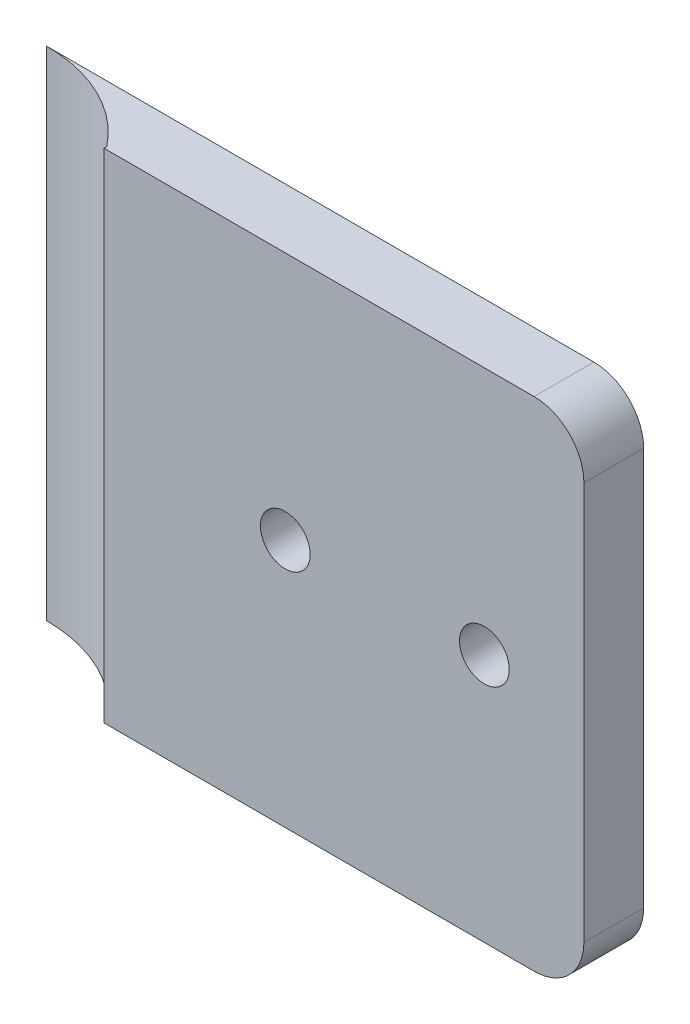
from build123d import *

# Parameters (mm, degrees)
BOSS_EXTRUDE1_DEPTH   = 6
BOSS_EXTRUDE2_DEPTH   = 50
M6_TAPPED_HOLE1_D     = 5
M6_TAPPED_HOLE1_DEPTH = 15
M6_TAPPED_HOLE1_TIP   = 1.502151548


with BuildPart() as part:
    # Sketch1 → Boss-Extrude1 (new body)
    with BuildSketch(Plane.XY.offset(-15)):
        with BuildLine():
            Line((11.8, -5), (55, -5))
            ThreePointArc((55, -5), (58.535533906, -6.464466094), (60, -10))
            Line((60, -10), (60, -50))
            ThreePointArc((60, -50), (58.535533906, -53.535533906), (55, -55))
            Line((55, -55), (11.8, -55))
            Line((11.8, -55), (11.8, -5))
        make_face()
    extrude(amount=BOSS_EXTRUDE1_DEPTH)

    # Sketch2 → Boss-Extrude2 (add)
    with BuildSketch(Plane(origin=(0, -5, 0), x_dir=(1, 0, 0), z_dir=(0, 1, 0))):
        with BuildLine():
            Line((0, 15), (11.8, 15))
            Line((11.8, 15), (11.8, 9.260669522))
            ThreePointArc((11.8, 9.260669522), (6.560867213, 13.489070443), (0, 15))
        make_face()
    extrude(amount=-BOSS_EXTRUDE2_DEPTH)

    # M6 Tapped Hole1
    with Locations(Plane(origin=(50, -30, -9), x_dir=(1, 0, 0), z_dir=(0, 0, 1))):
        with Locations((0, 0), (-20, 0)):
            Hole(M6_TAPPED_HOLE1_D / 2, depth=M6_TAPPED_HOLE1_DEPTH)
            with Locations((0, 0, -(M6_TAPPED_HOLE1_DEPTH + M6_TAPPED_HOLE1_TIP / 2))):  # 118° drill point
                Cone(0, M6_TAPPED_HOLE1_D / 2, M6_TAPPED_HOLE1_TIP, mode=Mode.SUBTRACT)


solid = part.part
